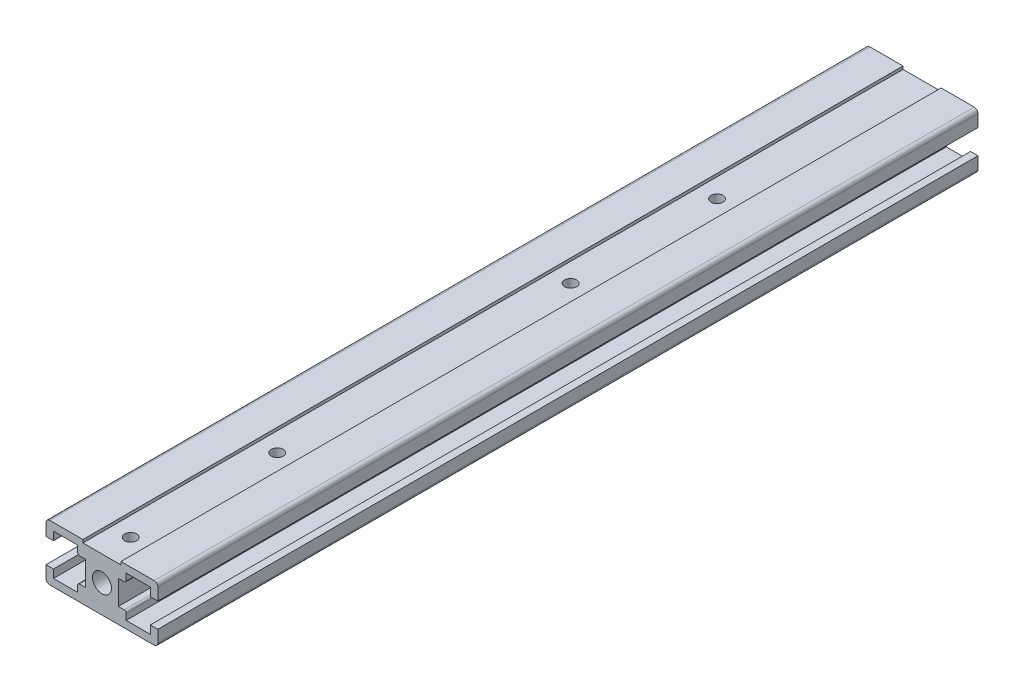
from build123d import *

# Parameters (mm, degrees)
SKETCH_1_W             = 30
SKETCH_1_H             = 15
EXTRUDE_1_DEPTH        = 220
FILLET_1_R             = 1
SKETCH_2_R             = 2.55
CUT_EXTRUDE_1_DEPTH    = 230
SKETCH_3_W             = 21.2
SKETCH_3_H             = 6.55
CUT_EXTRUDE_2_DEPTH    = 230
SKETCH_4_W             = 6.5
SKETCH_4_H             = 11
CUT_EXTRUDE_3_DEPTH    = 230
FILLET_2_R             = 0.5
SKETCH_5_R             = 1.6
CUT_EXTRUDE_4_DEPTH    = 10
PATTERN_LINEAR_1_COUNT = 2
PATTERN_LINEAR_1_PITCH = 118
SKETCH_7_W             = 10.2
SKETCH_7_H             = 220
CUT_EXTRUDE_6_DEPTH    = 0.8


with BuildPart() as part:
    # 草图1 → 凸台-拉伸1 (new body)
    with BuildSketch(Plane.XY):
        Rectangle(SKETCH_1_W, SKETCH_1_H)
    extrude(amount=EXTRUDE_1_DEPTH)

    # 圆角1
    fillet_1_edges = [part.edges().sort_by_distance(p)[0] for p in [
        (15, -7.5, 110),
        (-15, -7.5, 110),
        (-15, 7.5, 110),
        (15, 7.5, 110),
    ]]
    fillet(fillet_1_edges, radius=FILLET_1_R)

    # 草图2 → 切除-拉伸1 (cut)
    with BuildSketch(Plane.XY.offset(220)):
        Circle(SKETCH_2_R)
    extrude(amount=-CUT_EXTRUDE_1_DEPTH, mode=Mode.SUBTRACT)

    # 草图3 → 切除-拉伸2 (cut)
    with BuildSketch(Plane.XY.offset(220)):
        with Locations((-15, -0.025)):
            Rectangle(SKETCH_3_W, SKETCH_3_H)
    cut_extrude_2 = extrude(amount=-CUT_EXTRUDE_2_DEPTH, mode=Mode.SUBTRACT)

    # 镜向1: 切除-拉伸2 across plane
    add(cut_extrude_2.mirror(Plane(origin=(0, 0, 0), x_dir=(0, 0, 1), z_dir=(1, 0, 0))), mode=Mode.SUBTRACT)

    # 草图4 → 切除-拉伸3 (cut)
    with BuildSketch(Plane.XY.offset(220)):
        with Locations((-9.75, 0)):
            Rectangle(SKETCH_4_W, SKETCH_4_H)
    cut_extrude_3 = extrude(amount=-CUT_EXTRUDE_3_DEPTH, mode=Mode.SUBTRACT)

    # 镜向2: 切除-拉伸3 across plane
    add(cut_extrude_3.mirror(Plane(origin=(0, 0, 0), x_dir=(0, 0, 1), z_dir=(1, 0, 0))), mode=Mode.SUBTRACT)

    # 圆角2
    fillet_2_edges = [part.edges().sort_by_distance(p)[0] for p in [
        (6.5, -3.3, 110),
        (6.5, 3.25, 110),
        (-6.5, 3.25, 110),
        (-6.5, -3.3, 110),
    ]]
    fillet(fillet_2_edges, radius=FILLET_2_R)

    # 草图5 → 切除-拉伸4 (cut)
    with BuildSketch(Plane(origin=(0, 7.5, 0), x_dir=(1, 0, 0), z_dir=(0, 1, 0))):
        with Locations(Location((0, -55, 0), (0, 0, 270))):
            Circle(SKETCH_5_R)
        with Locations(Location((0, -94.285714286, 0), (0, 0, 270))):
            Circle(SKETCH_5_R)
    cut_extrude_4 = extrude(amount=-CUT_EXTRUDE_4_DEPTH, mode=Mode.SUBTRACT)

    # 阵列(线性)1: 切除-拉伸4 ×2
    with Locations(*[(0, 0, i * PATTERN_LINEAR_1_PITCH) for i in range(1, PATTERN_LINEAR_1_COUNT)]):
        add(cut_extrude_4, mode=Mode.SUBTRACT)

    # 草图7 → 切除-拉伸6 (cut)
    with BuildSketch(Plane(origin=(0, 7.5, 0), x_dir=(1, 0, 0), z_dir=(0, 1, 0))):
        with Locations((0, -110)):
            Rectangle(SKETCH_7_W, SKETCH_7_H)
    extrude(amount=-CUT_EXTRUDE_6_DEPTH, mode=Mode.SUBTRACT)


solid = part.part
